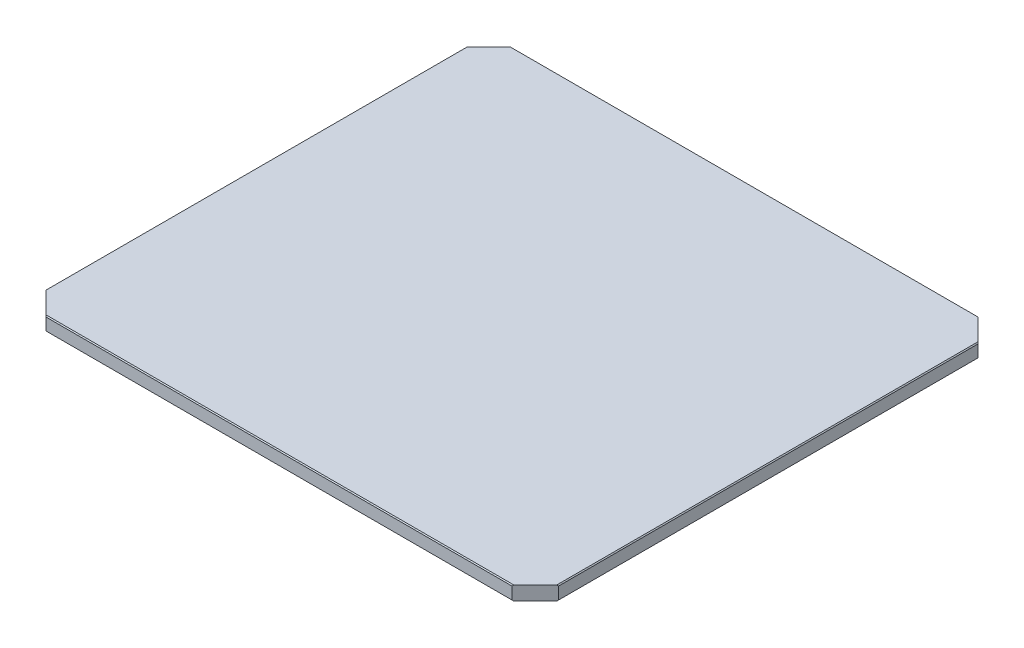
SolidWorks part; units mm, degrees
material "橡胶海绵"
ref_plane "前视基准面" through (0, 0, 0) normal (0, 0, 1) x (1, 0, 0)
ref_plane "上视基准面" through (0, 0, 0) normal (0, 1, 0) x (1, 0, 0)
ref_plane "右视基准面" through (0, 0, 0) normal (1, 0, 0) x (0, 0, -1)
sketch "Sketch1" plane through (0, 0, 0) normal (0, 1, 0) x (1, 0, 0)
  line L1 (55, -50) -> (-55, -50)
  line L2 (55, -50) -> (55, 50)
  line L3 (55, 50) -> (-55, 50)
  line L4 (-55, -50) -> (-55, 50)
  line L5 (55, -50) -> (-55, 50) construction
  line L6 (55, 50) -> (-55, -50) construction
  point P0 (0, 0)
  dimension "D1" = 110
  dimension "D2" = 100
extrude "Extrude1" add sketch "Sketch1" along normal blind 3
hole_wizard "CBORE for M4 Hex Socket Head Cap Screw1" positions "Sketch3" profile "Sketch2" counterbore size "M4" standard "ISO"
sketch "Sketch3" plane through (0, 0, 0) normal (0, -1, 0) x (-1, 0, 0)
  point P0 (40, -40)
  point P3 (-40, -40)
  point P6 (-40, 40)
  point P9 (40, 40)
sketch "Sketch2" plane through (-40, 0, 40) normal (1, 0, 0) x (0, 0, -1)
  line L0 (0, 0) -> (0, 3)
  line L1 (0, 3) -> (2.25, 3)
  line L3 (2.25, 3) -> (2.25, 4.4)
  line L4 (2.25, 4.4) -> (4, 4.4)
  line L5 (4, 4.4) -> (4, 0)
  line L7 (4, 0) -> (0, 0)
  line L11 (0, -6.35) -> (0, 107.95) construction
  dimension "通孔孔直径" = 4.5
  dimension "通孔孔深度" = 3
  dimension "柱形沉头孔直径" = 8
  dimension "柱形沉头孔深度" = 4.4
chamfer "Chamfer1" distance 5 angle 45 4 edges at (-55, 1.5, 50) (-55, 1.5, -50) (55, 1.5, -50) (55, 1.5, 50)
chamfer "Chamfer2" distance 0.2 angle 45 8 edges at (-55, 0, 0) (0, 0, -50) (0, 0, 50) (55, 0, 0) (55, 3, 0) (0, 3, -50) (-55, 3, 0) (0, 3, 50)
